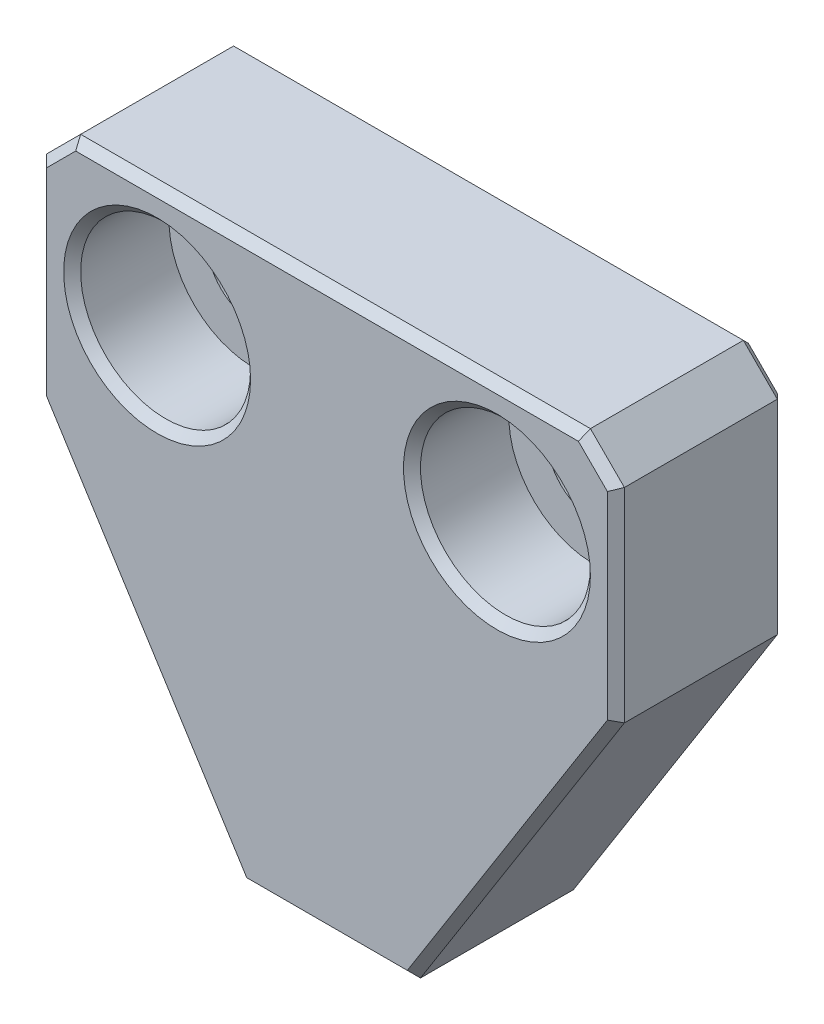
from build123d import *

# Parameters (mm, degrees)
SKETCH1_W                                            = 34
SKETCH1_H                                            = 14
BOSS_EXTRUDE1_DEPTH                                  = 10
HOLE_SIZE_PER_SOCKET_HEAD_CAP_SCREW_TYPE_D           = 5.5
HOLE_SIZE_PER_SOCKET_HEAD_CAP_SCREW_TYPE_CBORE_D     = 10
HOLE_SIZE_PER_SOCKET_HEAD_CAP_SCREW_TYPE_CBORE_DEPTH = 5.7
BOSS_EXTRUDE2_DEPTH                                  = 10
CHAMFER2_SIZE                                        = 2
CHAMFER1_SIZE                                        = 0.5


with BuildPart() as part:
    # Sketch1 → Boss-Extrude1 (new body)
    with BuildSketch(Plane.XY):
        Rectangle(SKETCH1_W, SKETCH1_H)
    extrude(amount=BOSS_EXTRUDE1_DEPTH)

    # Hole size per socket head cap screw type1 (through all)
    with Locations(Plane(origin=(-10, 0, 10), x_dir=(1, 0, 0), z_dir=(0, 0, 1))):
        with Locations((0, 0), (20, 0)):
            CounterBoreHole(HOLE_SIZE_PER_SOCKET_HEAD_CAP_SCREW_TYPE_D / 2, HOLE_SIZE_PER_SOCKET_HEAD_CAP_SCREW_TYPE_CBORE_D / 2, HOLE_SIZE_PER_SOCKET_HEAD_CAP_SCREW_TYPE_CBORE_DEPTH)

    # Sketch3 → Boss-Extrude2 (add)
    with BuildSketch(Plane.XY.offset(10)):
        Polygon((-17, -7), (-5, -26), (5, -26), (17, -7), align=None)
    extrude(amount=-BOSS_EXTRUDE2_DEPTH)

    # Chamfer2
    chamfer2_edges = [part.edges().sort_by_distance(p)[0] for p in [
        (-17, 7, 5),
        (17, 7, 5),
    ]]
    chamfer(chamfer2_edges, length=CHAMFER2_SIZE)

    # Chamfer1
    chamfer1_edges = [part.edges().sort_by_distance(p)[0] for p in [
        (17, -1, 10),
        (5, 0, 10),
        (12.75, 0, 0),
        (-15, 0, 10),
        (-7.25, 0, 0),
        (-11, -16.5, 10),
        (0, -26, 10),
        (11, -16.5, 10),
        (11, -16.5, 0),
        (0, -26, 0),
        (-11, -16.5, 0),
        (-17, -1, 0),
        (-17, -1, 10),
        (0, 7, 0),
        (16, 6, 0),
        (-16, 6, 0),
        (0, 7, 10),
        (16, 6, 10),
        (-16, 6, 10),
        (17, -1, 0),
    ]]
    chamfer(chamfer1_edges, length=CHAMFER1_SIZE)


solid = part.part
